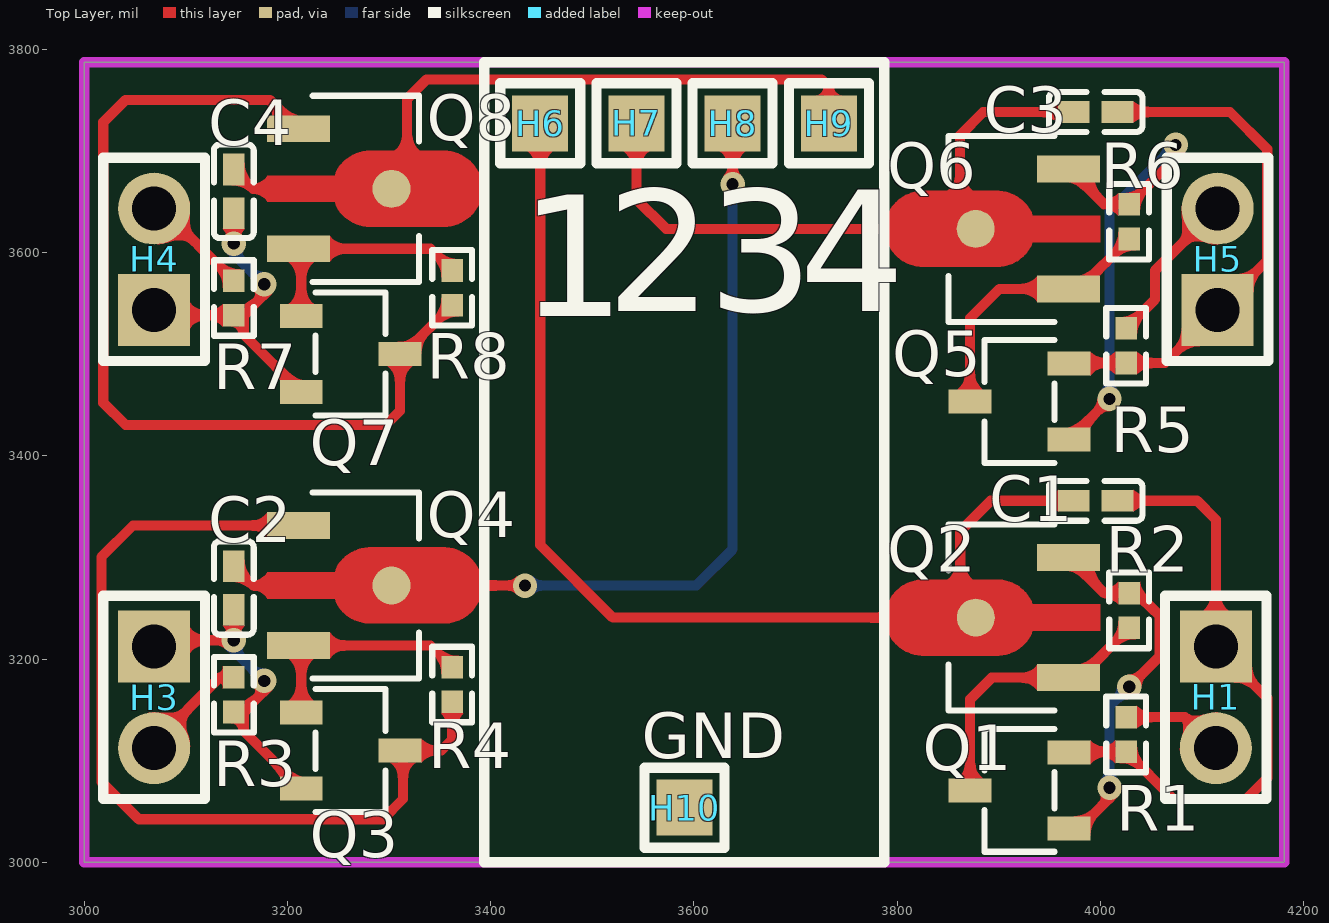
[diagram p0: Top Layer view]
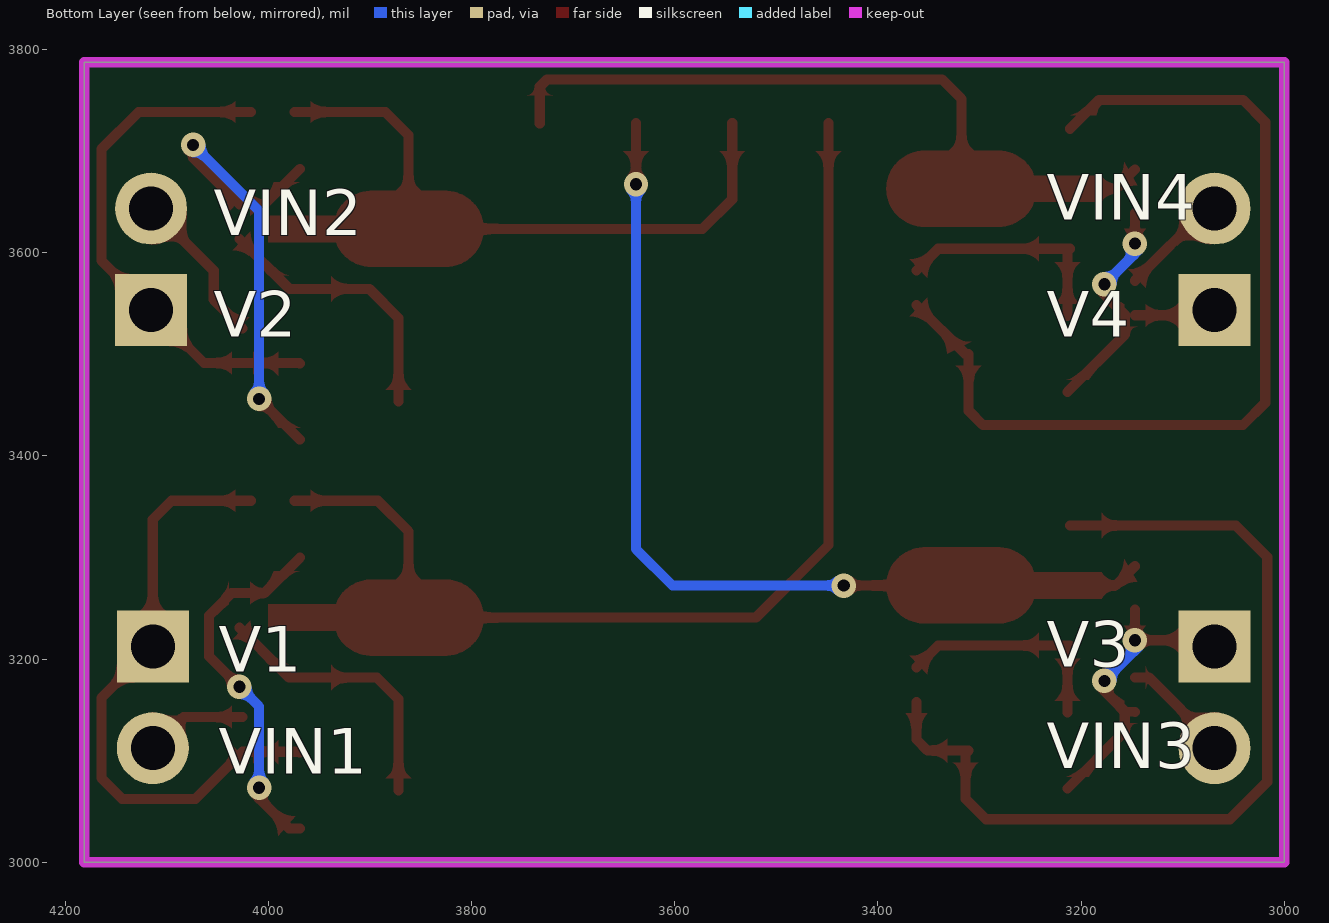
[diagram p1: Bottom Layer view, seen from below]
# Altium PCB MISC51650.pcbdoc
Units mil, origin at the board's own origin, x right, y up, seen from the top; angles counter-clockwise.
Board outline 1181.1 x 787.4 mil, 2 copper layers (Top Layer, Bottom Layer), stack 62.206 mil thick; 29 components, 21 nets, 61 pads, 10 vias.

## Layer stack, top to bottom
Top Solder Mask Layer: solder mask 0.394, Dk 3.3
Top Layer: signal copper 1.379
Dielectric1: surface 59.449, FR4, Dk 4.5
Bottom Layer: signal copper 1.378
Bottom Solder Mask Layer: solder mask 0.394, Dk 3.3

## Board outline
4181.1,3787.4 3000,3787.4 3000,3000 4181.1,3000

## Design rules (kind name [scope] priority, off if disabled: settings)
BoardOutlineClearance copperThickness2oz_1 [All] p2 off: genericclearance=7.99 ignorepadtopadclearanceinfootprint=FALSE except(0: Arc-SplitContinuation Track-SplitContinuation SMDPad-SplitContinuation THPad-SplitContinuation Via-SplitContinuation Fill-SplitContinuation Region-SplitContinuation Poly-SplitContinuation Text-SplitContinuation Hole-SplitContinuation; 5.98: Arc-CutoutEdge Track-CutoutEdge SMDPad-CutoutEdge THPad-CutoutEdge Via-CutoutEdge Text-CutoutEdge; 6.9: Hole-OutlineEdge Hole-CutoutEdge; 10: Poly-OutlineEdge Poly-CutoutEdge; 11.81: Arc-OutlineEdge Track-OutlineEdge SMDPad-OutlineEdge THPad-OutlineEdge Via-OutlineEdge Fill-OutlineEdge Region-OutlineEdge Text-OutlineEdge Fill-CutoutEdge Region-CutoutEdge)
BoardOutlineClearance Plane_innerPlane_1 [All] p4 off: genericclearance=4.02 ignorepadtopadclearanceinfootprint=FALSE except(0: Arc-SplitContinuation Track-SplitContinuation SMDPad-SplitContinuation THPad-SplitContinuation Via-SplitContinuation Fill-SplitContinuation Region-SplitContinuation Poly-SplitContinuation Text-SplitContinuation Hole-SplitContinuation; 5.98: Arc-CutoutEdge Track-CutoutEdge SMDPad-CutoutEdge THPad-CutoutEdge Via-CutoutEdge Text-CutoutEdge; 6.9: Hole-OutlineEdge Hole-CutoutEdge; 10: Poly-OutlineEdge Poly-CutoutEdge; 11.81: Arc-OutlineEdge Track-OutlineEdge SMDPad-OutlineEdge THPad-OutlineEdge Via-OutlineEdge Fill-OutlineEdge Region-OutlineEdge Text-OutlineEdge Fill-CutoutEdge Region-CutoutEdge)
BoardOutlineClearance Copper_copperRegion_1 [All] p6 off: genericclearance=4.02 ignorepadtopadclearanceinfootprint=FALSE except(0: Arc-SplitContinuation Track-SplitContinuation SMDPad-SplitContinuation THPad-SplitContinuation Via-SplitContinuation Fill-SplitContinuation Region-SplitContinuation Poly-SplitContinuation Text-SplitContinuation Hole-SplitContinuation; 5.98: Arc-CutoutEdge Track-CutoutEdge SMDPad-CutoutEdge THPad-CutoutEdge Via-CutoutEdge Text-CutoutEdge; 6.9: Hole-OutlineEdge Hole-CutoutEdge; 10: Poly-OutlineEdge Poly-CutoutEdge; 11.81: Arc-OutlineEdge Track-OutlineEdge SMDPad-OutlineEdge THPad-OutlineEdge Via-OutlineEdge Fill-OutlineEdge Region-OutlineEdge Text-OutlineEdge Fill-CutoutEdge Region-CutoutEdge)
BoardOutlineClearance copperThickness1oz_1 [All] p8: genericclearance=4.02 ignorepadtopadclearanceinfootprint=FALSE except(0: Arc-SplitContinuation Track-SplitContinuation SMDPad-SplitContinuation THPad-SplitContinuation Via-SplitContinuation Fill-SplitContinuation Region-SplitContinuation Poly-SplitContinuation Text-SplitContinuation Hole-SplitContinuation; 5.98: Arc-CutoutEdge Track-CutoutEdge SMDPad-CutoutEdge THPad-CutoutEdge Via-CutoutEdge Text-CutoutEdge; 6.9: Hole-OutlineEdge Hole-CutoutEdge; 10: Poly-OutlineEdge Poly-CutoutEdge; 11.81: Arc-OutlineEdge Track-OutlineEdge SMDPad-OutlineEdge THPad-OutlineEdge Via-OutlineEdge Fill-OutlineEdge Region-OutlineEdge Text-OutlineEdge Fill-CutoutEdge Region-CutoutEdge)
Clearance copperThickness2oz [All] p1 off: gap=7.99 ignorepadtopadclearanceinfootprint=FALSE except(5.98: SMDPad-Track SMDPad-SMDPad THPad-Track SMDPad-THPad THPad-THPad Track-Via SMDPad-Via THPad-Via Via-Via Fill-SMDPad Region-SMDPad Fill-THPad Region-THPad Fill-Via Region-Via Fill-Fill Fill-Region Region-Region Arc-Track Arc-SMDPad Arc-THPad Arc-Via Fill-Arc Region-Arc Arc-Arc Text-Track SMDPad-Text Text-THPad Text-Via Fill-Text Region-Text Arc-Text Text-Text; 6.9: Hole-Track Hole-SMDPad Hole-THPad Hole-Via Fill-Hole Region-Hole Hole-Arc Hole-Text; 10: Poly-Track Poly-SMDPad Poly-THPad Poly-Via Poly-Fill Poly-Region Poly-Poly Poly-Arc Poly-Text Poly-Hole; 11.81: Fill-Track Region-Track)
Clearance Plane_innerPlane [All] p3 off: gap=4.02 ignorepadtopadclearanceinfootprint=FALSE except(5.98: SMDPad-Track SMDPad-SMDPad THPad-Track SMDPad-THPad THPad-THPad Track-Via SMDPad-Via THPad-Via Via-Via Fill-SMDPad Region-SMDPad Fill-THPad Region-THPad Fill-Via Region-Via Fill-Fill Fill-Region Region-Region Arc-Track Arc-SMDPad Arc-THPad Arc-Via Fill-Arc Region-Arc Arc-Arc Text-Track SMDPad-Text Text-THPad Text-Via Fill-Text Region-Text Arc-Text Text-Text; 6.9: Hole-Track Hole-SMDPad Hole-THPad Hole-Via Fill-Hole Region-Hole Hole-Arc Hole-Text; 10: Poly-Track Poly-SMDPad Poly-THPad Poly-Via Poly-Fill Poly-Region Poly-Poly Poly-Arc Poly-Text Poly-Hole; 11.81: Fill-Track Region-Track)
Clearance Copper_copperRegion [All] p5 off: gap=4.02 ignorepadtopadclearanceinfootprint=FALSE except(5.98: SMDPad-Track SMDPad-SMDPad THPad-Track SMDPad-THPad THPad-THPad Track-Via SMDPad-Via THPad-Via Via-Via Fill-SMDPad Region-SMDPad Fill-THPad Region-THPad Fill-Via Region-Via Fill-Fill Fill-Region Region-Region Arc-Track Arc-SMDPad Arc-THPad Arc-Via Fill-Arc Region-Arc Arc-Arc Text-Track SMDPad-Text Text-THPad Text-Via Fill-Text Region-Text Arc-Text Text-Text; 6.9: Hole-Track Hole-SMDPad Hole-THPad Hole-Via Fill-Hole Region-Hole Hole-Arc Hole-Text; 10: Poly-Track Poly-SMDPad Poly-THPad Poly-Via Poly-Fill Poly-Region Poly-Poly Poly-Arc Poly-Text Poly-Hole; 11.81: Fill-Track Region-Track)
Clearance copperThickness1oz [All] p7: gap=4.02 ignorepadtopadclearanceinfootprint=FALSE except(5.98: SMDPad-Track SMDPad-SMDPad THPad-Track SMDPad-THPad THPad-THPad Track-Via SMDPad-Via THPad-Via Via-Via Fill-SMDPad Region-SMDPad Fill-THPad Region-THPad Fill-Via Region-Via Fill-Fill Fill-Region Region-Region Arc-Track Arc-SMDPad Arc-THPad Arc-Via Fill-Arc Region-Arc Arc-Arc Text-Track SMDPad-Text Text-THPad Text-Via Fill-Text Region-Text Arc-Text Text-Text; 6.9: Hole-Track Hole-SMDPad Hole-THPad Hole-Via Fill-Hole Region-Hole Hole-Arc Hole-Text; 10: Poly-Track Poly-SMDPad Poly-THPad Poly-Via Poly-Fill Poly-Region Poly-Poly Poly-Arc Poly-Text Poly-Hole; 11.81: Fill-Track Region-Track)
DiffPairsRouting differentialPair [All] p1: maxlimit=6 minlimit=6 mostfreqgap=6 toplayer_minwidth=5 toplayer_prefwidth=10 toplayer_maxwidth=100 toplayer_mingap=6 toplayer_prefgap=6 toplayer_maxgap=6 bottomlayer_minwidth=5 bottomlayer_prefwidth=10 bottomlayer_maxwidth=100 bottomlayer_mingap=6 bottomlayer_prefgap=6 bottomlayer_maxgap=6 maxuncoupledlength=10
HoleToHoleClearance otherClearance [All] p1: gap=11.81 allowstackedmicrovias=TRUE
Length netLength [All] p1: minlimit=0 maxlimit=0
PasteMaskExpansion pasteMaskExpansion [All] p1: expansion=0
PlaneConnect innerPlane [All] p1: planeconnectstyle=Relief reliefexpansion=20 reliefentries=4 reliefconductorwidth=10 reliefairgap=10
PolygonConnect copperRegion [All] p1: connectstyle=Relief reliefconductorwidth=10 reliefentries=4 polygonreliefangle="90 Angle" airgapwidth=10 via.connectstyle=Relief via.reliefconductorwidth=10 via.reliefentries=4 via.polygonreliefangle="90 Angle" via.airgapwidth=10
RoutingVias viaSize [All] p1: holewidth=12.01 width=24.02 viastyle="Through Hole" minholewidth=11.81 minwidth=19.68 maxholewidth=248.03 maxwidth=393.7
SolderMaskExpansion solderMaskExpansion [IsVia] p1: expansion=-1000 istentingtop=TRUE
SolderMaskExpansion solderMaskExpansion [All] p2: expansion=2 istentingtop=FALSE
Width copperThickness2oz_2 [All] p1 off: maxlimit=100 minlimit=8 preferedwidth=10
Width copperThickness1oz_2 [All] p2: maxlimit=100 minlimit=5 preferedwidth=10

## Components (designator, comment, footprint, x,y, rotation, side; value= is the part's Value field where it differs from the comment)
C1 "1nF" C0402 3995.47,3355.85 r0 top
C2 "1nF" C0402 3147.11,3270 r270 top
C3 "1nF" C0402 3995.43,3738.48 r0 top
C4 "1nF" C0402 3147.11,3660.43 r270 top
H1 "" HDR-TH_2P-P2.54-V-M-1 4113.7,3162.4 r270 top
H3 "" HDR-TH_2P-P2.54-V-M-1 3068.7,3162.4 r270 top
H4 "" HDR-TH_2P-P2.54-V-M-1 3068.7,3593.48 r90 top
H5 "" HDR-TH_2P-P2.54-V-M-1 4115.43,3593.48 r90 top
H6 "" HDR-TH_1P-V-M_XKB_X4611WV-01I-C28D40 3448.7,3727.4 r0 top
H7 "" HDR-TH_1P-V-M_XKB_X4611WV-01I-C28D40 3543.4,3727.4 r0 top
H8 "" HDR-TH_1P-V-M_XKB_X4611WV-01I-C28D40 3638.1,3727.4 r0 top
H9 "" HDR-TH_1P-V-M_XKB_X4611WV-01I-C28D40 3732.8,3727.4 r0 top
H10 "" HDR-TH_1P-V-M_XKB_X4611WV-01I-C28D40 3590.75,3053.78 r0 top
Q1 "BC856B" SOT-23-3_L2.9-W1.6-P1.90-LS2.8-BR 3920.47,3070.85 r0 top
Q2 "2N2222AU" SOT-89-3_L4.5-W2.4-P1.50-LS4.0-BR 3915.47,3240.85 r0 top
Q3 "BC856B" SOT-23-3_L2.9-W1.6-P1.90-LS2.8-BR 3262.11,3110 r180 top
Q4 "2N2222AU" SOT-89-3_L4.5-W2.4-P1.50-LS4.0-BR 3264.33,3272.5 r180 top
Q5 "BC856B" SOT-23-3_L2.9-W1.6-P1.90-LS2.8-BR 3920.43,3453.48 r0 top
Q6 "2N2222AU" SOT-89-3_L4.5-W2.4-P1.50-LS4.0-BR 3915.43,3623.48 r0 top
Q7 "BC856B" SOT-23-3_L2.9-W1.6-P1.90-LS2.8-BR 3262.11,3500.43 r180 top
Q8 "2N2222AU" SOT-89-3_L4.5-W2.4-P1.50-LS4.0-BR 3264.33,3662.93 r180 top
R1 "3.9K" R0402 4025.47,3125.85 r270 top
R2 "200k" R0402 4028.43,3247.89 r90 top
R3 "3.9K" R0402 3147.11,3165 r270 top
R4 "200k" R0402 3362.11,3175 r90 top
R5 "3.9K" R0402 4025.43,3508.48 r270 top
R6 "200k" R0402 4028.39,3630.52 r90 top
R7 "3.9K" R0402 3147.11,3555.43 r270 top
R8 "200k" R0402 3362.11,3565.43 r90 top

## Footprints (in the part's own frame and the unit in brackets; to place one, negate y for a bottom-side part, rotate by r counter-clockwise, add the part's x,y. Pads: shape width x height; smd on the part's side, far side on the other; paste and mask are expansions set on the pad)
C0402 [mm]
  rect 0.79x0.54 smd paste-100 mask+0.051: 1(-0.545,0) 2(0.545,0)
  silkscreen extent -1.17,-0.5 1.17,0.5
HDR-TH_1P-V-M_XKB_X4611WV-01I-C28D40 [mm]
  rect 1.4x1.4 smd: 1(0,0)
  silkscreen extent -1,-1 1,1
HDR-TH_2P-P2.54-V-M-1 [mm]
  rect 1.8x1.8 hole 1.1: 1(-1.27,0)
  round 1.8 hole 1.1: 2(1.27,0)
  silkscreen extent -2.54,-1.27 2.54,1.27
R0402 [mm]
  rect 0.566x0.54 smd paste-100 mask+0.051: 1(-0.433,0) 2(0.433,0)
  silkscreen extent -0.94,-0.5 0.94,0.5
SOT-23-3_L2.9-W1.6-P1.90-LS2.8-BR [mm]
  rect 1.07x0.6 smd: 1(1.235,-0.95) 2(1.235,0.95) 3(-1.235,0)
  silkscreen extent -0.88,-1.54 0.88,1.54
SOT-89-3_L4.5-W2.4-P1.50-LS4.0-BR [mm]
  rect 1.575x0.672 smd: 1(1.356,-1.5) 3(1.356,1.5)
  round 0.95 smd: 2(-0.966,0)
  Top Layer region: -2.283,0.95 -0.429,0.95 -0.384,0.949 -0.34,0.946 -0.296,0.941 -0.252,0.933 -0.208,0.924 -0.165,0.913 -0.123,0.899 -0.081,0.884 -0.04,0.867 0,0.847 0.04,0.826 0.078,0.804 0.115,0.779 0.151,0.753 0.185,0.725 0.219,0.695 0.251,0.664 0.281,0.631 0.31,0.597 0.337,0.562 0.362,0.525 0.386,0.488 0.408,0.449 0.428,0.409 0.447,0.33 2.144,0.33 2.144,-0.33 0.447,-0.33 0.428,-0.409 0.408,-0.449 0.386,-0.488 0.362,-0.525 0.337,-0.562 0.31,-0.597 0.281,-0.631 0.251,-0.664 0.219,-0.695 0.185,-0.725 0.151,-0.753 0.115,-0.779 0.078,-0.804 0.04,-0.826 0,-0.847 -0.04,-0.867 -0.081,-0.884 -0.123,-0.899 -0.165,-0.913 -0.208,-0.924 -0.252,-0.933 -0.296,-0.941 -0.34,-0.946 -0.384,-0.949 -0.429,-0.95 -2.283,-0.95 -2.328,-0.949 -2.372,-0.946 -2.416,-0.941 -2.46,-0.933 -2.504,-0.924 -2.547,-0.913 -2.589,-0.899 -2.631,-0.884 -2.672,-0.867 -2.712,-0.847 -2.752,-0.826 -2.79,-0.804 -2.827,-0.779 -2.863,-0.753 -2.898,-0.725 -2.931,-0.695 -2.963,-0.664 -2.993,-0.631 -3.022,-0.597 -3.049,-0.562 -3.075,-0.525 -3.098,-0.488 -3.12,-0.449 -3.14,-0.409 -3.159,-0.369 -3.175,-0.327 -3.189,-0.285 -3.202,-0.242 -3.212,-0.199 -3.22,-0.155 -3.227,-0.111 -3.231,-0.067 -3.233,-0.022 -3.233,0.022 -3.231,0.067 -3.227,0.111 -3.22,0.155 -3.212,0.199 -3.202,0.242 -3.189,0.285 -3.175,0.327 -3.159,0.369 -3.14,0.409 -3.12,0.449 -3.098,0.488 -3.075,0.525 -3.049,0.562 -3.022,0.597 -2.993,0.631 -2.963,0.664 -2.931,0.695 -2.898,0.725 -2.863,0.753 -2.827,0.779 -2.79,0.804 -2.752,0.826 -2.712,0.847 -2.672,0.867 -2.631,0.884 -2.589,0.899 -2.547,0.913 -2.504,0.924 -2.46,0.933 -2.416,0.941 -2.372,0.946 -2.328,0.949
  silkscreen extent -1.65,-2.33 1,2.33

## Via types
v1: diameter 24.02, hole 12, Top Layer to Bottom Layer, 10 vias

## Nets (pads, with @x,y where several pads share a name; then routed paths per layer and width w, separated by ;. In a path a pad name is that pad's centre, name@x,y a point inside that pad or via, vN(x,y) a via of type N, cw(c..) or ccw(c..) an arc to the next point about the centre after c; other vN are vias at no path point)
$1N629: Q1.3 Q2.1 R2.1 | length 275.4
  Top Layer w10: Q1.3 3871.84,3160.54 3893.1,3181.8 Q2.1 3979.38,3181.8 R2.1
$1N634: Q1.1 Q2.3 R2.2 | length 365.7
  Top Layer w10: Q2.3 4003.85,3264.93 R2.2 4036.28,3264.93 4058.43,3242.78 4058.43,3202.78 v1(4028.43,3172.78) ; Q1.1 3979.59,3033.45 4009.09,3062.95 v1(4009.09,3073.45)
  Bottom Layer w10: v1(4009.09,3073.45) 4009.09,3153.45 v1(4028.43,3172.78)
$1N1172: Q3.3 Q4.1 R4.1 | length 890.5
  Top Layer w10: Q4.1 3047.85,3331.55 3016.81,3300.51 3016.81,3079.29 3053.7,3042.4 3293.7,3042.4 3313.7,3062.4 3313.7,3107.03 Q3.3 3351.3,3110 3362.11,3120.81 R4.1
$1N1177: Q3.1 Q4.3 R4.2 | length 227.1
  Top Layer w10: Q3.1 3213.48,3210.89 Q4.3 3340.7,3213.44 R4.2
$1N1509: Q5.3 Q6.1 R6.1 | length 270.9
  Top Layer w10: Q5.3 3871.8,3535.5 3900.73,3564.43 Q6.1 3979.34,3564.43 R6.1
$1N1514: Q5.1 Q6.3 R6.2 | length 485
  Top Layer w10: Q6.3 4003.81,3647.56 R6.2 4074.05,3693.23 v1(4074.05,3706.08) ; Q5.1 v1(4009.05,3456.08)
  Bottom Layer w10: v1(4009.05,3456.08) 4009.05,3641.08 v1(4074.05,3706.08)
$1N1525: Q7.3 Q8.1 R8.1 | length 923.3
  Top Layer w10: Q8.1 3182.48,3750.43 3040.73,3750.43 3018.7,3728.4 3018.7,3452.4 3040.67,3430.43 3296.73,3430.43 3310.73,3444.43 Q7.3 3314.15,3500.43 R8.1
$1N1530: Q7.1 Q8.3 R8.2 | length 227.1
  Top Layer w10: Q7.1 3213.48,3601.32 Q8.3 3340.7,3603.87 R8.2
GND: H10.1
V1: C1.2 H1.1 Q1.2 R1.2 | length 603
  Top Layer w10: Q1.2 3969.65,3108.81 R1.2 4071.88,3062.4 4143.7,3062.4 4164.29,3082.99 4164.29,3161.81 H1.1 4113.7,3337.4 4095.25,3355.85 C1.2
V2: C3.2 H5.1 Q5.2 R5.2 | length 509.3
  Top Layer w10: Q5.2 3969.61,3491.44 R5.2 4063.39,3491.44 H5.1 4164.29,3592.35 4164.29,3701.81 4127.62,3738.48 C3.2
V3: C2.2 H3.1 Q3.2 R3.2 | length 311
  Top Layer w10: H3.1 3074.84,3218.54 v1(3147.11,3218.54) C2.2 ; R3.2 R3.2@3157.11,3148.54 ; v1(3177.11,3178.54) 3177.11,3168.54 R3.2@3157.11,3148.54 ; Q3.2 3157.11,3128.97 R3.2@3157.11,3148.54
  Bottom Layer w10: v1(3147.11,3218.54) 3147.11,3208.54 v1(3177.11,3178.54)
V4: C4.2 H4.1 Q7.2 R7.2 | length 300.5
  Top Layer w10: H4.1 3073.79,3538.39 R7.2 ; v1(3147.11,3608.97) C4.2 ; v1(3177.11,3568.97) 3177.11,3558.97 3157.11,3538.97 3157.11,3519.4 Q7.2
  Bottom Layer w10: v1(3147.11,3608.97) 3147.11,3598.97 v1(3177.11,3568.97)
VIN1: H1.2 R1.1 | length 100.9
  Top Layer w10: R1.1 4083.21,3142.89 H1.2
VIN2: H5.2 R5.1 | length 155.6
  Top Layer w10: R5.1 4053.7,3553.8 4053.7,3582.4 4114.78,3643.48 H5.2
VIN3: H3.2 R3.1 | length 110.2
  Top Layer w10: H3.2 3068.7,3117.4 3133.34,3182.04 R3.1
VIN4: H4.2 R7.1 | length 107.8
  Top Layer w10: H4.2 3076.09,3643.48 R7.1
VOUT1: C1.1 H6.1 Q2.2 | length 1067.3
  Top Layer w10: H6.1 3448.7,3312.4 3520.26,3240.84 3862.07,3240.84 3862.07,3325.77 3892.15,3355.85 C1.1
VOUT2: C3.1 H7.1 Q6.2 | length 619.1
  Top Layer w10: H7.1 3543.4,3652.7 3572.63,3623.47 3862.03,3623.47 3862.03,3715.73 3884.78,3738.48 C3.1
VOUT3: C2.1 H8.1 Q4.2 | length 932.9
  Top Layer w10: C2.1 3166.05,3272.51 3317.73,3272.51 3413.59,3272.51 3413.7,3272.4 v1(3433.7,3272.4) ; v1(3638.1,3667.4) H8.1
  Bottom Layer w10: v1(3433.7,3272.4) 3602.22,3272.4 3638.1,3308.27 v1(3638.1,3667.4)
VOUT4: C4.1 H9.1 Q8.2 | length 728.9
  Top Layer w10: C4.1 3166.05,3662.94 3317.73,3662.94 3317.73,3751.43 3336.89,3770.59 3725.51,3770.59 3732.8,3763.31 H9.1

## Keep-outs
Board Outline Layer:
  the board outline again, w10

## Other copper
Top Layer:
  region net V1: 4047.48,3360.85 4047.48,3350.85 4043.41,3350.48 4039.47,3349.4 4035.79,3347.62 4032.48,3345.22 4032.48,3366.48 4035.79,3364.08 4039.47,3362.3 4043.41,3361.22 4047.48,3360.85
  region net VOUT1: 3943.46,3350.85 3943.46,3360.85 3947.53,3361.22 3951.47,3362.3 3955.15,3364.08 3958.46,3366.48 3958.46,3345.22 3955.15,3347.62 3951.47,3349.4 3947.53,3350.48 3943.46,3350.85
  region net V3: 3152.11,3218.54 3142.11,3218.54 3141.74,3222.48 3140.65,3226.29 3138.87,3229.83 3136.48,3232.99 3157.74,3232.99 3155.34,3229.83 3153.56,3226.29 3152.47,3222.48 3152.11,3218.54
  region net VOUT3: 3163.04,3282.6 3160.89,3270.6 3157.29,3272.88 3153.37,3274.55 3149.23,3275.56 3144.98,3275.91 3157.74,3298.51 3158.08,3294.26 3159.1,3290.12 3160.76,3286.2 3163.04,3282.6
  region net V2: 4047.44,3743.48 4047.44,3733.48 4043.37,3733.12 4039.43,3732.03 4035.74,3730.26 4032.44,3727.85 4032.44,3749.11 4035.74,3746.71 4039.43,3744.94 4043.37,3743.85 4047.44,3743.48
  region net VOUT2: 3943.41,3733.48 3943.41,3743.48 3947.48,3743.85 3951.42,3744.94 3955.11,3746.71 3958.41,3749.11 3958.41,3727.85 3955.11,3730.26 3951.42,3732.03 3947.48,3733.12 3943.41,3733.48
  region net V4: 3152.11,3608.97 3142.11,3608.97 3141.74,3612.91 3140.65,3616.72 3138.87,3620.26 3136.48,3623.42 3157.74,3623.42 3155.34,3620.26 3153.56,3616.72 3152.47,3612.91 3152.11,3608.97
  region net VOUT4: 3163.04,3673.03 3160.89,3661.03 3157.29,3663.31 3153.37,3664.98 3149.23,3665.99 3144.98,3666.34 3157.74,3688.94 3158.08,3684.69 3159.1,3680.55 3160.76,3676.63 3163.04,3673.03
  region net $1N634: 3989.63,3050.56 3995.46,3042.25 3993.19,3038.65 3991.52,3034.73 3990.5,3030.59 3990.16,3026.34 3973.72,3045.26 3977.97,3045.6 3982.11,3046.62 3986.03,3048.29 3989.63,3050.56
  region net V1: 4005.16,3113.81 4005.16,3103.81 4001.71,3103.49 3998.39,3102.56 3995.28,3101.03 3992.51,3098.97 3990.16,3096.44 3990.16,3120.06 3992.68,3117.89 3995.52,3116.14 3998.59,3114.86 4001.83,3114.07 4005.16,3113.81
  region net $1N629: 3866.84,3097.66 3876.84,3097.66 3877.17,3094.2 3878.12,3090.86 3879.67,3087.76 3881.77,3084.99 3884.34,3082.66 3859.34,3082.66 3861.92,3084.99 3864.02,3087.76 3865.57,3090.86 3866.52,3094.2 3866.84,3097.66
  region net $1N634: 4002.49,3273.36 3982.92,3278.79 3979.99,3281.38 3976.76,3283.57 3973.28,3285.35 3969.6,3286.68 3994.6,3286.68 3995.93,3283.01 3997.71,3279.52 3999.91,3276.29 4002.49,3273.36
  region net $1N629: 3922.87,3176.8 3922.87,3186.8 3926.33,3187.12 3929.66,3188.08 3932.77,3189.63 3935.54,3191.73 3937.87,3194.3 3937.87,3169.3 3935.54,3171.87 3932.77,3173.97 3929.66,3175.52 3926.33,3176.48 3922.87,3176.8
  region net $1N629: 3993.43,3202.92 4010.38,3205.73 4005.1,3200.41 3999.88,3195.03 3980.11,3195.03 3983.78,3196.36 3987.26,3198.14 3990.5,3200.33 3993.43,3202.92
  region net $1N1177: 3208.48,3174.21 3218.48,3174.21 3218.8,3170.75 3219.76,3167.41 3221.31,3164.31 3223.41,3161.54 3225.98,3159.21 3200.98,3159.21 3203.55,3161.54 3205.65,3164.31 3207.21,3167.41 3208.16,3170.75 3208.48,3174.21
  region net V3: 3182.9,3096.11 3200.85,3092.3 3203.78,3089.72 3207.01,3087.52 3210.49,3085.74 3214.17,3084.41 3192.42,3084.41 3187.96,3090.5 3182.9,3096.11
  region net $1N1172: 3318.7,3083.19 3308.7,3083.19 3308.38,3086.65 3307.43,3089.99 3305.87,3093.09 3303.77,3095.86 3301.2,3098.19 3326.2,3098.19 3323.63,3095.86 3321.53,3093.09 3319.98,3089.99 3319.02,3086.65 3318.7,3083.19
  region net $1N1172: 3346.79,3115 3346.79,3105 3343.41,3104.71 3340.13,3103.85 3337.04,3102.45 3334.24,3100.54 3331.79,3098.19 3331.79,3121.81 3334.24,3119.46 3337.04,3117.55 3340.13,3116.15 3343.41,3115.29
  region net $1N1177: 3218.48,3185.21 3208.48,3185.21 3208.16,3188.67 3207.21,3192.01 3205.65,3195.12 3203.55,3197.88 3200.98,3200.21 3225.98,3200.21 3223.41,3197.88 3221.31,3195.12 3219.76,3192.01 3218.8,3188.67 3218.48,3185.21
  region net $1N1177: 3256.93,3218.44 3256.93,3208.44 3253.48,3208.12 3250.14,3207.17 3247.03,3205.61 3244.27,3203.52 3241.93,3200.94 3241.93,3225.94 3244.27,3223.37 3247.03,3221.27 3250.14,3219.72 3253.48,3218.76 3256.93,3218.44
  region net $1N1172: 3164.93,3326.55 3164.93,3336.55 3168.38,3336.87 3171.72,3337.83 3174.83,3339.38 3177.59,3341.48 3179.93,3344.05 3179.93,3319.05 3177.59,3321.63 3174.83,3323.72 3171.72,3325.28 3168.38,3326.23 3164.93,3326.55
  region net $1N1514: 3981.68,3435.79 3999.63,3439.59 3994.57,3433.99 3990.11,3427.89 3968.36,3427.89 3972.04,3429.22 3975.52,3431 3978.75,3433.2 3981.68,3435.79
  region net V2: 4005.11,3496.44 4005.11,3486.44 4001.67,3486.13 3998.34,3485.19 3995.24,3483.67 3992.47,3481.6 3990.11,3479.07 3990.11,3502.69 3992.64,3500.52 3995.48,3498.77 3998.55,3497.49 4001.79,3496.71 4005.11,3496.44
  region net $1N1509: 3866.8,3480.29 3876.8,3480.29 3877.12,3476.84 3878.08,3473.5 3879.63,3470.39 3881.73,3467.63 3884.3,3465.29 3859.3,3465.29 3861.87,3467.63 3863.97,3470.39 3865.53,3473.5 3866.48,3476.84 3866.8,3480.29
  region net $1N1514: 4002.45,3655.99 3982.88,3661.42 3979.95,3664.01 3976.71,3666.21 3973.23,3667.99 3969.56,3669.31 3994.56,3669.31 3995.89,3665.64 3997.66,3662.16 3999.86,3658.93 4002.45,3655.99
  region net $1N1509: 3922.82,3559.43 3922.82,3569.43 3926.28,3569.75 3929.62,3570.71 3932.73,3572.26 3935.49,3574.36 3937.82,3576.93 3937.82,3551.93 3935.49,3554.51 3932.73,3556.61 3929.62,3558.16 3926.28,3559.11 3922.82,3559.43
  region net $1N1509: 3993.38,3585.55 4010.34,3588.37 4005.06,3583.04 3999.83,3577.66 3980.06,3577.66 3983.74,3578.99 3987.22,3580.77 3990.45,3582.97 3993.38,3585.55
  region net $1N1530: 3208.48,3564.64 3218.48,3564.64 3218.8,3561.18 3219.76,3557.84 3221.31,3554.74 3223.41,3551.97 3225.98,3549.64 3200.98,3549.64 3203.55,3551.97 3205.65,3554.74 3207.21,3557.84 3208.16,3561.18 3208.48,3564.64
  region net V4: 3182.9,3486.54 3200.85,3482.73 3203.78,3480.15 3207.01,3477.95 3210.49,3476.17 3214.17,3474.84 3192.42,3474.84 3187.96,3480.93 3182.9,3486.54
  region net $1N1525: 3324.19,3517.54 3337.1,3516.31 3334.82,3512.71 3333.15,3508.79 3332.14,3504.65 3331.79,3500.4 3308.28,3512.24 3312.53,3512.58 3316.66,3513.6 3320.59,3515.27 3324.19,3517.54
  region net $1N1525: 3315.73,3473.62 3305.73,3473.62 3305.41,3477.08 3304.46,3480.42 3302.9,3483.52 3300.8,3486.29 3298.23,3488.62 3323.23,3488.62 3320.66,3486.29 3318.56,3483.52 3317.01,3480.42 3316.05,3477.08 3315.73,3473.62
  region net $1N1530: 3218.48,3575.64 3208.48,3575.64 3208.16,3579.1 3207.21,3582.44 3205.65,3585.55 3203.55,3588.31 3200.98,3590.64 3225.98,3590.64 3223.41,3588.31 3221.31,3585.55 3219.76,3582.44 3218.8,3579.1 3218.48,3575.64
  region net $1N1530: 3256.93,3608.87 3256.93,3598.87 3253.48,3598.55 3250.14,3597.6 3247.03,3596.04 3244.27,3593.95 3241.93,3591.37 3241.93,3616.37 3244.27,3613.8 3247.03,3611.7 3250.14,3610.15 3253.48,3609.19 3256.93,3608.87
  region net $1N1525: 3178.95,3746.89 3196.88,3743.1 3199.81,3740.52 3203.04,3738.32 3206.53,3736.54 3210.2,3735.21 3185.2,3735.21 3184.3,3738.45 3182.94,3741.52 3181.14,3744.35 3178.95,3746.89
  region net V1: 4041.4,3099.95 4034.84,3092.37 4031.23,3094.65 4027.31,3096.31 4023.17,3097.33 4018.93,3097.68 4036.1,3115.86 4036.44,3111.61 4037.46,3107.47 4039.13,3103.55 4041.4,3099.95
  region net V1: 3999.84,3103.81 3999.84,3113.81 4003.15,3114.07 4006.38,3114.83 4009.45,3116.09 4012.3,3117.81 4014.84,3119.95 4014.84,3097.68 4012.3,3099.81 4009.45,3101.53 4006.38,3102.79 4003.15,3103.55 3999.84,3103.81
  region net VIN1: 4051.1,3147.89 4051.1,3137.89 4047.79,3137.63 4044.56,3136.87 4041.48,3135.61 4038.64,3133.89 4036.1,3131.76 4036.1,3154.03 4038.64,3151.89 4041.48,3150.17 4044.56,3148.91 4047.79,3148.15 4051.1,3147.89
  region net $1N634: 4046.25,3262.04 4050.31,3243.83 4044.84,3248.98 4039.06,3253.8 4039.06,3276.07 4040.01,3272.18 4041.55,3268.49 4043.65,3265.08 4046.25,3262.04
  region net $1N634: 4003.85,3259.93 4003.85,3269.93 4006.97,3270.19 4010.01,3270.96 4012.88,3272.22 4015.5,3273.94 4017.8,3276.07 4017.8,3253.8 4015.5,3255.92 4012.88,3257.64 4010.01,3258.9 4006.97,3259.67 4003.85,3259.93
  region net $1N629: 4019.06,3214.41 4012.5,3221.99 4014.77,3225.59 4016.44,3229.51 4017.46,3233.65 4017.8,3237.9 4034.97,3219.72 4030.72,3219.37 4026.59,3218.35 4022.66,3216.69 4019.06,3214.41
  region net V3: 3162.11,3128.97 3152.11,3128.97 3151.74,3131.34 3150.69,3133.48 3149.04,3135.2 3146.95,3136.36 3144.61,3136.82 3157.74,3136.82 3158.03,3134.5 3158.9,3132.33 3160.29,3130.45 3162.11,3128.97
  region net V3: 3169.77,3168.27 3165.71,3150.07 3163.12,3147.15 3160.91,3143.93 3159.11,3140.48 3157.74,3136.82 3157.74,3159.09 3162.01,3161.79 3166.04,3164.86 3169.77,3168.27
  region net VIN3: 3133.34,3177.04 3133.34,3187.04 3135.02,3188.72 3136.1,3190.83 3136.48,3193.18 3136.48,3170.91 3136.1,3173.25 3135.02,3175.36 3133.34,3177.04
  region net $1N1177: 3346.17,3200.9 3352.74,3208.48 3356.34,3206.2 3360.26,3204.54 3364.4,3203.52 3368.65,3203.18 3351.48,3184.99 3351.13,3189.24 3350.11,3193.38 3348.45,3197.3 3346.17,3200.9
  region net $1N1172: 3367.11,3131.82 3357.11,3131.82 3356.74,3135.9 3355.65,3139.84 3353.88,3143.52 3351.48,3146.82 3372.74,3146.82 3370.33,3143.52 3368.56,3139.84 3367.47,3135.9 3367.11,3131.82
  region net V2: 4051.06,3496.44 4051.06,3486.44 4047.74,3486.19 4044.51,3485.42 4041.44,3484.16 4038.6,3482.44 4036.06,3480.31 4036.06,3502.58 4038.6,3500.44 4041.44,3498.72 4044.51,3497.47 4047.74,3496.7 4051.06,3496.44
  region net V2: 3999.8,3486.44 3999.8,3496.44 4003.11,3496.7 4006.34,3497.47 4009.41,3498.72 4012.25,3500.44 4014.8,3502.58 4014.8,3480.31 4012.25,3482.44 4009.41,3484.16 4006.34,3485.42 4003.11,3486.19 3999.8,3486.44
  region net VIN2: 4034.79,3541.96 4041.36,3534.39 4039.08,3530.78 4037.42,3526.86 4036.4,3522.72 4036.06,3518.48 4018.88,3536.66 4023.13,3537 4027.27,3538.02 4031.19,3539.69 4034.79,3541.96
  region net $1N1514: 4003.81,3642.56 4003.81,3652.56 4006.93,3652.82 4009.97,3653.59 4012.83,3654.85 4015.45,3656.57 4017.76,3658.7 4017.76,3636.43 4015.45,3638.55 4012.83,3640.27 4009.97,3641.53 4006.93,3642.3 4003.81,3642.56
  region net $1N1514: 4037.75,3664 4044.32,3656.43 4042.04,3652.82 4040.38,3648.9 4039.36,3644.76 4039.02,3640.52 4021.84,3658.7 4026.09,3659.04 4030.23,3660.06 4034.15,3661.73 4037.75,3664
  region net $1N1509: 4019.02,3597.04 4012.45,3604.62 4014.73,3608.22 4016.39,3612.15 4017.41,3616.28 4017.76,3620.53 4034.93,3602.35 4030.68,3602.01 4026.54,3600.99 4022.62,3599.32 4019.02,3597.04
  region net V4: 3162.11,3519.4 3152.11,3519.4 3151.74,3521.76 3150.69,3523.91 3149.04,3525.63 3146.95,3526.78 3144.61,3527.25 3157.74,3527.25 3158.03,3524.93 3158.9,3522.76 3160.29,3520.88 3162.11,3519.4
  region net V4: 3121.48,3533.39 3121.48,3543.39 3124.79,3543.65 3128.02,3544.41 3131.09,3545.67 3133.93,3547.39 3136.48,3549.52 3136.48,3527.25 3133.93,3529.39 3131.09,3531.11 3128.02,3532.37 3124.79,3533.13 3121.48,3533.39
  region net V4: 3169.77,3558.7 3165.71,3540.5 3163.12,3537.58 3160.91,3534.36 3159.11,3530.91 3157.74,3527.25 3157.74,3549.52 3162.01,3552.22 3166.04,3555.29 3169.77,3558.7
  region net VIN4: 3131.17,3581.33 3137.74,3588.91 3141.34,3586.63 3145.26,3584.97 3149.4,3583.95 3153.65,3583.6 3136.48,3565.42 3136.13,3569.67 3135.11,3573.81 3133.45,3577.73 3131.17,3581.33
  region net $1N1530: 3346.17,3591.33 3352.74,3598.91 3356.34,3596.63 3360.26,3594.97 3364.4,3593.95 3368.65,3593.6 3351.48,3575.42 3351.13,3579.67 3350.11,3583.81 3348.45,3587.73 3346.17,3591.33
  region net $1N1525: 3352.74,3531.95 3346.17,3539.53 3348.45,3543.13 3350.11,3547.05 3351.13,3551.19 3351.48,3555.44 3368.65,3537.25 3364.4,3536.91 3360.26,3535.89 3356.34,3534.23 3352.74,3531.95
  region net VOUT1: 3453.7,3684.84 3443.7,3684.84 3443.38,3688.3 3442.43,3691.64 3440.87,3694.74 3438.77,3697.51 3436.2,3699.84 3461.2,3699.84 3458.63,3697.51 3456.53,3694.74 3454.98,3691.64 3454.02,3688.3 3453.7,3684.84
  region net VOUT2: 3548.4,3684.84 3538.4,3684.84 3538.08,3688.3 3537.12,3691.64 3535.57,3694.74 3533.47,3697.51 3530.9,3699.84 3555.9,3699.84 3553.33,3697.51 3551.23,3694.74 3549.67,3691.64 3548.72,3688.3 3548.4,3684.84
  region net VOUT3: 3643.1,3684.84 3633.1,3684.84 3632.78,3688.3 3631.82,3691.64 3630.27,3694.74 3628.17,3697.51 3625.6,3699.84 3650.6,3699.84 3648.02,3697.51 3645.92,3694.74 3644.37,3691.64 3643.42,3688.3 3643.1,3684.84
  region net VOUT4: 3727.8,3763.31 3737.8,3763.31 3738.15,3760.88 3739.19,3758.67 3740.83,3756.85 3742.92,3755.57 3745.3,3754.96 3720.3,3754.96 3722.67,3755.57 3724.76,3756.85 3726.4,3758.67 3727.44,3760.88 3727.8,3763.31
  region net VIN1: 4079.68,3139.35 4086.75,3146.43 4087.94,3145.5 4089.32,3144.85 4090.88,3144.45 4092.59,3144.27 4094.43,3144.28 4096.37,3144.45 4100.44,3145.12 4108.74,3146.96 4112.57,3147.62 4114.31,3147.77 4115.92,3147.77 4078.34,3110.18 4078.33,3111.79 4078.48,3113.54 4079.14,3117.36 4080.98,3125.66 4081.65,3129.74 4081.82,3131.67 4081.83,3133.51 4081.65,3135.22 4081.25,3136.78 4080.61,3138.17
  region net V1: 4154.44,3178.74 4147.37,3171.67 4143.76,3173.94 4139.84,3175.61 4135.7,3176.63 4131.46,3176.97 4149.13,3194.65 4149.48,3190.4 4150.49,3186.26 4152.16,3182.34 4154.44,3178.74
  region net V1: 4108.7,3262.83 4118.7,3262.83 4119.02,3259.38 4119.98,3256.04 4121.53,3252.93 4123.63,3250.17 4126.2,3247.83 4101.2,3247.83 4103.77,3250.17 4105.87,3252.93 4107.43,3256.04 4108.38,3259.38 4108.7,3262.83
  region net VIN3: 3094.82,3150.59 3105.64,3147.27 3103.82,3145.26 3102.41,3143.33 3101.39,3141.44 3100.71,3139.59 3100.33,3137.76 3100.2,3135.93 3100.3,3134.07 3100.56,3132.19 3101.46,3128.24 3102.57,3123.94 3103.56,3119.15 3103.91,3116.52 3104.11,3113.72 3062.96,3147.37 3066.54,3147.66 3070.69,3147.6 3079.8,3147.2 3084.3,3147.24 3088.46,3147.7 3090.33,3148.13 3092.04,3148.75 3093.54,3149.56
  region net V3: 3119.13,3223.54 3119.13,3213.54 3115.68,3213.22 3112.34,3212.26 3109.23,3210.71 3106.47,3208.61 3104.13,3206.04 3104.13,3231.04 3106.47,3228.47 3109.23,3226.37 3112.34,3224.82 3115.68,3223.86 3119.13,3223.54
  region net VIN4: 3107.09,3619.56 3105.56,3606.94 3103.59,3608.73 3101.66,3610.11 3099.77,3611.12 3097.89,3611.81 3096.02,3612.21 3094.13,3612.36 3092.22,3612.29 3090.28,3612.04 3086.22,3611.16 3081.85,3610.03 3077.05,3608.93 3074.46,3608.49 3071.72,3608.18 3103.35,3650.89 3103.63,3649.17 3103.79,3647.29 3103.83,3643.19 3103.54,3634.31 3103.61,3629.95 3104.09,3625.9 3104.55,3624.05 3105.18,3622.37 3106.02,3620.86
  region net V4: 3119.13,3543.39 3119.13,3533.39 3115.68,3533.07 3112.34,3532.11 3109.23,3530.56 3106.47,3528.46 3104.13,3525.89 3104.13,3550.89 3106.47,3548.32 3109.23,3546.22 3112.34,3544.66 3115.68,3543.71 3119.13,3543.39
  region net VIN2: 4084.29,3605.92 4077.7,3613.47 4078.68,3614.71 4079.45,3616.21 4080.03,3617.94 4080.44,3619.88 4080.85,3624.21 4080.84,3628.92 4080.27,3638.41 4080.05,3642.64 4080.09,3646.16 4117.19,3608.09 4114.28,3608.06 4111.6,3608.24 4109.13,3608.57 4106.84,3609.02 4102.69,3610.07 4098.97,3611 4097.2,3611.3 4095.47,3611.42 4093.74,3611.33 4091.99,3610.97 4090.19,3610.3 4088.33,3609.27 4086.37,3607.82
  region net V2: 4081.76,3502.75 4074.69,3509.82 4076.96,3513.42 4078.63,3517.34 4079.65,3521.48 4079.99,3525.73 4097.67,3508.05 4093.42,3507.71 4089.28,3506.69 4085.36,3505.02 4081.76,3502.75
  region net V2: 4149.09,3584.22 4156.16,3577.15 4153.89,3573.54 4152.22,3569.62 4151.2,3565.49 4150.86,3561.24 4133.18,3578.92 4137.43,3579.26 4141.57,3580.28 4145.49,3581.94 4149.09,3584.22
  region net VOUT1: 3773.68,3235.84 3773.68,3245.84 3781.2,3246.12 3788.68,3246.96 3788.52,3245.84 3788.52,3235.84 3788.68,3234.74 3781.2,3235.56 3773.68,3235.84
  region net VOUT1: 3857.07,3293.25 3867.07,3293.25 3867.39,3289.79 3868.35,3286.46 3869.9,3283.35 3872,3280.58 3874.57,3278.25 3867.07,3278.25 3857.07,3278.25 3849.57,3278.25 3852.14,3280.58 3854.24,3283.35 3855.8,3286.46 3856.75,3289.79 3857.07,3293.25
  region net VOUT3: 3406.12,3277.51 3406.12,3267.51 3398.6,3267.23 3391.12,3266.39 3391.28,3267.51 3391.28,3277.51 3391.12,3278.61 3398.6,3277.79 3406.12,3277.51
  region net VOUT3: 3166.05,3267.51 3166.05,3277.51 3169.32,3277.84 3172.46,3278.8 3175.34,3280.36 3177.87,3282.46 3179.93,3285.01 3179.93,3277.51 3179.93,3267.51 3179.93,3260.01 3177.87,3262.57 3175.34,3264.67 3172.46,3266.23 3169.32,3267.19 3166.05,3267.51
  region net VOUT2: 3773.64,3618.47 3773.64,3628.47 3781.16,3628.75 3788.64,3629.59 3788.48,3628.47 3788.48,3618.47 3788.64,3617.37 3781.16,3618.2 3773.64,3618.47
  region net VOUT2: 3857.03,3675.89 3867.03,3675.89 3867.35,3672.43 3868.3,3669.09 3869.86,3665.98 3871.96,3663.22 3874.53,3660.89 3867.03,3660.89 3857.03,3660.89 3849.53,3660.89 3852.1,3663.22 3854.2,3665.98 3855.75,3669.09 3856.71,3672.43 3857.03,3675.89
  region net VOUT4: 3166.05,3657.94 3166.05,3667.94 3169.32,3668.27 3172.46,3669.23 3175.34,3670.79 3177.87,3672.89 3179.93,3675.44 3179.93,3667.94 3179.93,3657.94 3179.93,3650.44 3177.87,3653 3175.34,3655.1 3172.46,3656.66 3169.32,3657.62 3166.05,3657.94
  region net VOUT4: 3312.73,3715.33 3322.73,3715.33 3323.05,3711.88 3324.01,3708.54 3325.56,3705.43 3327.66,3702.67 3330.23,3700.33 3322.73,3700.33 3312.73,3700.33 3305.23,3700.33 3307.8,3702.67 3309.9,3705.43 3311.46,3708.54 3312.41,3711.88 3312.73,3715.33
  region net $1N1514: 4001.03,3440.99 3993.95,3448.06 3994.7,3448.93 3995.32,3449.91 3996.24,3452.12 3996.8,3454.49 3997.07,3456.84 4009.8,3444.1 4007.46,3443.83 4005.08,3443.28 4002.88,3442.35 4001.89,3441.73
  region net $1N1514: 4079.05,3693.23 4069.05,3693.23 4068.96,3694.22 4068.71,3694.95 4068.31,3695.51 4067.8,3695.97 4066.52,3696.84 4065.04,3698.14 4083.06,3698.14 4081.59,3696.84 4080.3,3695.97 4079.79,3695.51 4079.39,3694.95 4079.14,3694.22
  region net $1N634: 4011.45,3058.24 3996.45,3057.38 3998.43,3059.49 3999.27,3060.57 3999.91,3061.66 4000.32,3062.77 4000.43,3063.89 4000.18,3065.04 3999.52,3066.2 4017.09,3064.49 4015.35,3062.79 4014.21,3061.43 4013.11,3060.04
  region net $1N634: 4036.45,3187.88 4043.52,3180.81 4042.78,3179.94 4042.16,3178.96 4041.24,3176.75 4040.68,3174.38 4040.41,3172.03 4027.68,3184.77 4030.02,3185.03 4032.4,3185.59 4034.6,3186.52 4035.58,3187.14
  region net V3: 3130.76,3213.54 3130.76,3223.54 3131.89,3223.63 3133.03,3223.88 3135.24,3224.79 3137.32,3226.07 3139.16,3227.55 3139.16,3209.53 3137.32,3211.01 3135.24,3212.29 3133.03,3213.2 3131.89,3213.45
  region net V3: 3142.11,3234.89 3152.11,3234.89 3152.2,3233.75 3152.45,3232.62 3153.36,3230.4 3154.64,3228.33 3156.11,3226.48 3138.1,3226.48 3139.57,3228.33 3140.85,3230.4 3141.76,3232.62 3142.02,3233.75
  region net V3: 3178.91,3163.27 3164.25,3162.76 3166.2,3164.85 3167.01,3165.92 3167.65,3167.01 3168.06,3168.12 3168.17,3169.26 3167.95,3170.41 3167.32,3171.58 3184.77,3169.3 3183.31,3167.95 3181.78,3166.35
  region net V4: 3142.11,3625.32 3152.11,3625.32 3152.2,3624.18 3152.45,3623.05 3153.36,3620.83 3154.64,3618.76 3156.11,3616.91 3138.1,3616.91 3139.57,3618.76 3140.85,3620.83 3141.76,3623.05 3142.02,3624.18
  region net V4: 3178.91,3553.7 3164.25,3553.19 3166.2,3555.28 3167.01,3556.35 3167.65,3557.44 3168.06,3558.55 3168.17,3559.69 3167.95,3560.84 3167.32,3562.01 3184.77,3559.73 3183.31,3558.38 3181.78,3556.78
  region net VOUT3: 3633.1,3683.75 3643.1,3683.75 3643.19,3682.61 3643.44,3681.48 3644.35,3679.26 3645.63,3677.19 3647.1,3675.34 3629.09,3675.34 3630.56,3677.19 3631.84,3679.26 3632.75,3681.48 3633.01,3682.61
  region net VOUT3: 3417.35,3267.4 3417.35,3277.4 3418.49,3277.49 3419.62,3277.75 3421.84,3278.65 3423.91,3279.94 3425.76,3281.41 3425.76,3263.4 3423.91,3264.87 3421.84,3266.15 3419.62,3267.06 3418.49,3267.31
Bottom Layer:
  region net $1N1514: 4004.05,3472.43 4014.05,3472.43 4014.14,3471.29 4014.39,3470.16 4015.3,3467.94 4016.59,3465.87 4018.06,3464.03 4000.04,3464.03 4001.52,3465.87 4002.8,3467.94 4003.71,3470.16 4003.96,3471.29
  region net $1N1514: 4066.03,3690.99 4058.95,3698.06 4059.7,3698.93 4060.32,3699.91 4061.24,3702.12 4061.8,3704.49 4062.07,3706.84 4074.8,3694.1 4072.46,3693.83 4070.08,3693.28 4067.88,3692.35 4066.89,3691.73
  region net $1N634: 4004.09,3089.8 4014.09,3089.8 4014.18,3088.66 4014.44,3087.53 4015.35,3085.31 4016.63,3083.24 4018.1,3081.39 4000.09,3081.39 4001.56,3083.24 4002.84,3085.31 4003.75,3087.53 4004,3088.66
  region net $1N634: 4020.4,3157.69 4013.33,3164.76 4014.07,3165.63 4014.7,3166.61 4015.62,3168.82 4016.18,3171.19 4016.44,3173.54 4029.18,3160.8 4026.84,3160.54 4024.46,3159.98 4022.25,3159.05 4021.27,3158.43
  region net V3: 3159.96,3202.76 3145.3,3203.27 3142.43,3206.35 3140.9,3207.95 3139.44,3209.3 3156.89,3211.58 3156.27,3210.41 3156.04,3209.26 3156.16,3208.12 3156.56,3207.01 3157.2,3205.92 3158.01,3204.85
  region net V3: 3162.01,3186.56 3169.08,3193.64 3169.95,3192.89 3170.93,3192.27 3173.14,3191.35 3175.51,3190.79 3177.86,3190.52 3165.12,3177.79 3164.86,3180.13 3164.3,3182.51 3163.37,3184.71 3162.75,3185.7
  region net V4: 3159.96,3593.19 3145.3,3593.7 3142.43,3596.78 3140.9,3598.38 3139.44,3599.73 3156.89,3602.01 3156.27,3600.84 3156.04,3599.69 3156.16,3598.55 3156.56,3597.44 3157.2,3596.35 3158.01,3595.28
  region net V4: 3162.01,3576.99 3169.08,3584.07 3169.95,3583.32 3170.93,3582.7 3173.14,3581.78 3175.51,3581.22 3177.86,3580.95 3165.12,3568.22 3164.86,3570.56 3164.3,3572.94 3163.37,3575.14 3162.75,3576.13
  region net VOUT3: 3643.1,3651.05 3633.1,3651.05 3633.01,3652.19 3632.75,3653.33 3631.84,3655.54 3630.56,3657.61 3629.09,3659.46 3647.1,3659.46 3645.63,3657.61 3644.35,3655.54 3643.44,3653.33 3643.19,3652.19
  region net VOUT3: 3450.05,3277.4 3450.05,3267.4 3448.91,3267.31 3447.78,3267.06 3445.56,3266.15 3443.49,3264.87 3441.64,3263.4 3441.64,3281.41 3443.49,3279.94 3445.56,3278.65 3447.78,3277.75 3448.91,3277.49

## Silkscreen, mask and mechanical layers (free items; w line width, h text height)
Top Silkscreen Layer:
  lines w10: 3393.7,3000 3393.7,3787.4 3787.4,3787.4 3787.4,3000 3393.7,3000
  text "2" at 3513.7,3542.4 h120
  text "3" at 3613.7,3542.4 h120
  text "4" at 3703.7,3542.4 h120
  text "1" at 3428.7,3537.4 h120
  text "GND" at 3548.7,3102.4 h45
Bottom Silkscreen Layer:
  text "VIN4" at 3233.7,3632.4 h45
  text "VIN2" at 4053.7,3617.4 h45
  text "V4" at 3233.7,3517.4 h45
  text "V2" at 4053.7,3517.4 h45
  text "V3" at 3233.7,3192.4 h45
  text "V1" at 4048.7,3187.4 h45
  text "VIN3" at 3233.7,3092.4 h45
  text "VIN1" at 4048.7,3087.4 h45